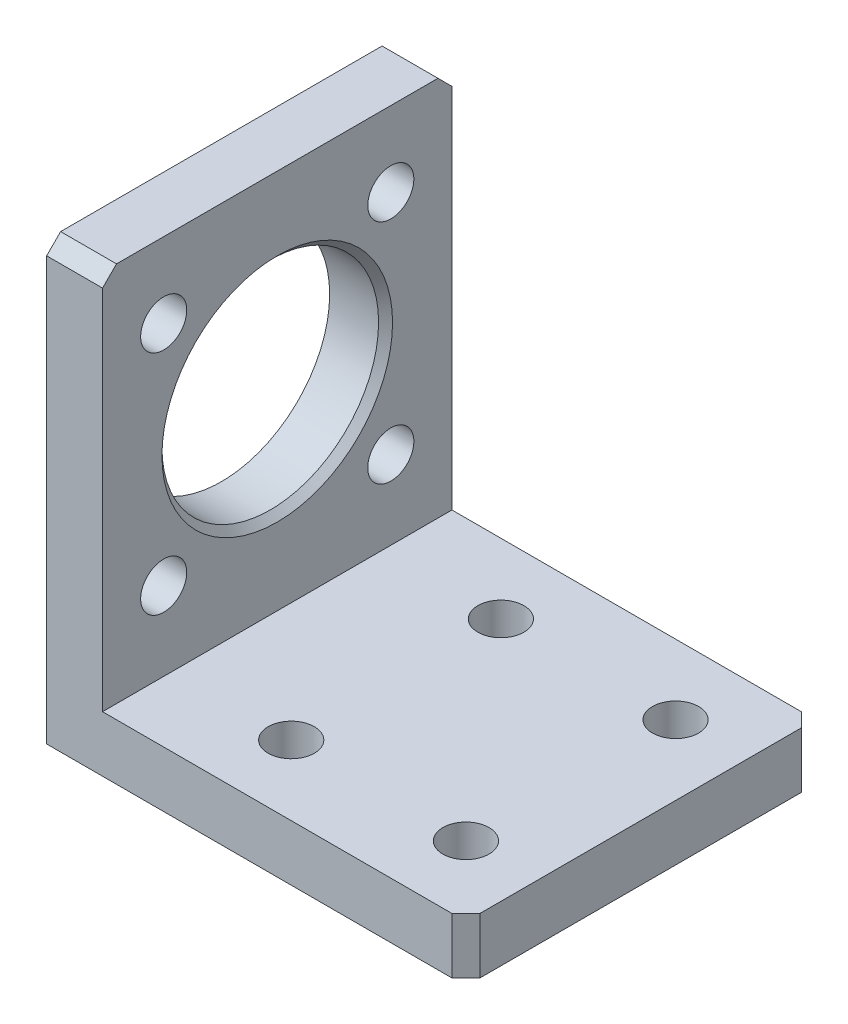
from build123d import *

# Parameters (mm, degrees)
BOSS_EXTRUDE1_DEPTH = 50
HOLE1_D             = 6.6
HOLE2_D             = 31
CHAMFER1_SIZE       = 1
CHAMFER2_SIZE       = 2
HOLE3_D             = 6.6


with BuildPart() as part:
    # Sketch1 → Boss-Extrude1 (new body)
    with BuildSketch(Plane.XY):
        Polygon((-40.819758101, 34.90625), (-40.819758101, -27.59375), (19.180241899, -27.59375), (19.180241899, -19.59375), (-32.819758101, -19.59375), (-32.819758101, 34.90625), align=None)
    extrude(amount=BOSS_EXTRUDE1_DEPTH)

    # Hole1 (through all)
    with Locations(Plane(origin=(-32.819758101, 0, 0), x_dir=(0, 0, -1), z_dir=(1, 0, 0))):
        with Locations((-41.25, 24.15625), (-8.75, 24.15625), (-8.75, -8.34375), (-41.25, -8.34375)):
            Hole(HOLE1_D / 2)

    # Hole2 (through all)
    with Locations(Plane(origin=(-32.819758101, 0, 0), x_dir=(0, 0, -1), z_dir=(1, 0, 0))):
        with Locations((-25, 7.90625)):
            Hole(HOLE2_D / 2)

    # Chamfer1
    chamfer1_edges = [part.edges().sort_by_distance(p)[0] for p in [
        (-32.819758101, 7.90625, 9.5),
    ]]
    chamfer(chamfer1_edges, length=CHAMFER1_SIZE)

    # Chamfer2
    chamfer2_edges = [part.edges().sort_by_distance(p)[0] for p in [
        (19.180241899, -23.59375, 50),
        (-36.819758101, 34.90625, 50),
        (19.180241899, -23.59375, 0),
        (-36.819758101, 34.90625, 0),
    ]]
    chamfer(chamfer2_edges, length=CHAMFER2_SIZE)

    # Hole3 (through all)
    with Locations(Plane(origin=(0, -19.59375, 0), x_dir=(1, 0, 0), z_dir=(0, 1, 0))):
        with Locations((-15.819758101, -40), (-15.819758101, -10), (9.180241899, -10), (9.180241899, -40)):
            Hole(HOLE3_D / 2)


solid = part.part
